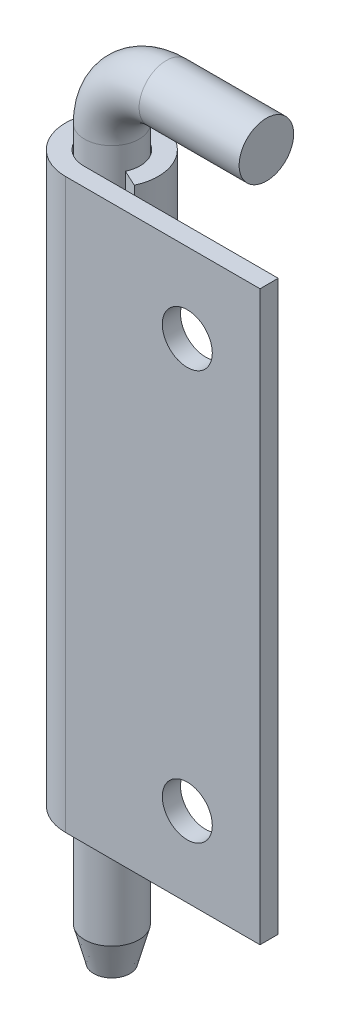
SolidWorks part; units mm, degrees
ref_plane "前视" through (0, 0, 0) normal (0, 0, 1) x (1, 0, 0)
ref_plane "上视" through (0, 0, 0) normal (0, 1, 0) x (1, 0, 0)
ref_plane "右视" through (0, 0, 0) normal (1, 0, 0) x (0, 0, -1)
sketch "草图1" plane through (0, 0, 0) normal (0, 0, 1) x (1, 0, 0)
  line L0 (0, 0) -> (0, 80)
  line L1 (6, 86) -> (17, 86)
  arc A0 (0, 80) -> (6, 86) centre (6, 80) cw
  point P6 (0, 86)
  dimension "D3" = 6
  dimension "D1" = 17
  dimension "D2" = 86
sketch "草图2" plane through (0, 0, 0) normal (0, 1, 0) x (1, 0, 0)
  circle A0 centre (0, 0) radius 3
  dimension "D1" = 6
sweep "扫描1" add profiles "草图2" path "草图1"
ref_plane "基准面1" through (0, 15, 0) normal (0, -1, 0) x (-1, 0, 0)
sketch "草图3" plane through (0, 15, 0) normal (0, -1, 0) x (-1, 0, 0)
  line L6 (0, 0) -> (-28.0181, 0) construction
  line L7 (0, 0) -> (-4.3836, -2.0441) construction
  line L8 (0, 0) -> (0, -2.8615) construction
  line L9 (-21.4, -3.1) -> (-21.4, -5.1)
  line L10 (-2.8096, -1.3101) -> (-4.6222, -2.1554)
  line L11 (0, -5.1) -> (-21.4, -5.1)
  line L12 (0, -3.1) -> (-21.4, -3.1)
  arc A2 (-4.6222, -2.1554) -> (0, -5.1) centre (0, 0) cw
  arc A5 (-2.8096, -1.3101) -> (0, -3.1) centre (0, 0) cw
  point P3 (0, 3.1)
  point P5 (-1.7443, 4.7924)
  point P6 (-1.0603, 2.913)
  point P8 (0, 5.1)
extrude "凸台-拉伸1" add sketch "草图3" against normal blind 62.5
sketch "草图5" plane through (0, 0, 3.1) normal (0, 0, 1) x (1, 0, 0)
  line L1 (21.4, 46.25) -> (-13.6129, 46.25) construction
  line L2 (21.4, 77.5) -> (21.4, 15) construction
  circle A0 centre (13.4, 23.75) radius 2.75
  circle A1 centre (13.4, 68.75) radius 2.75
  dimension "D1" = 8
  dimension "D2" = 45
  dimension "D3" = 5.5
extrude "切除-拉伸2" cut sketch "草图5" along normal through all
chamfer "倒角1" distance 1 angle 75 1 edges at (0, 0, 3)
